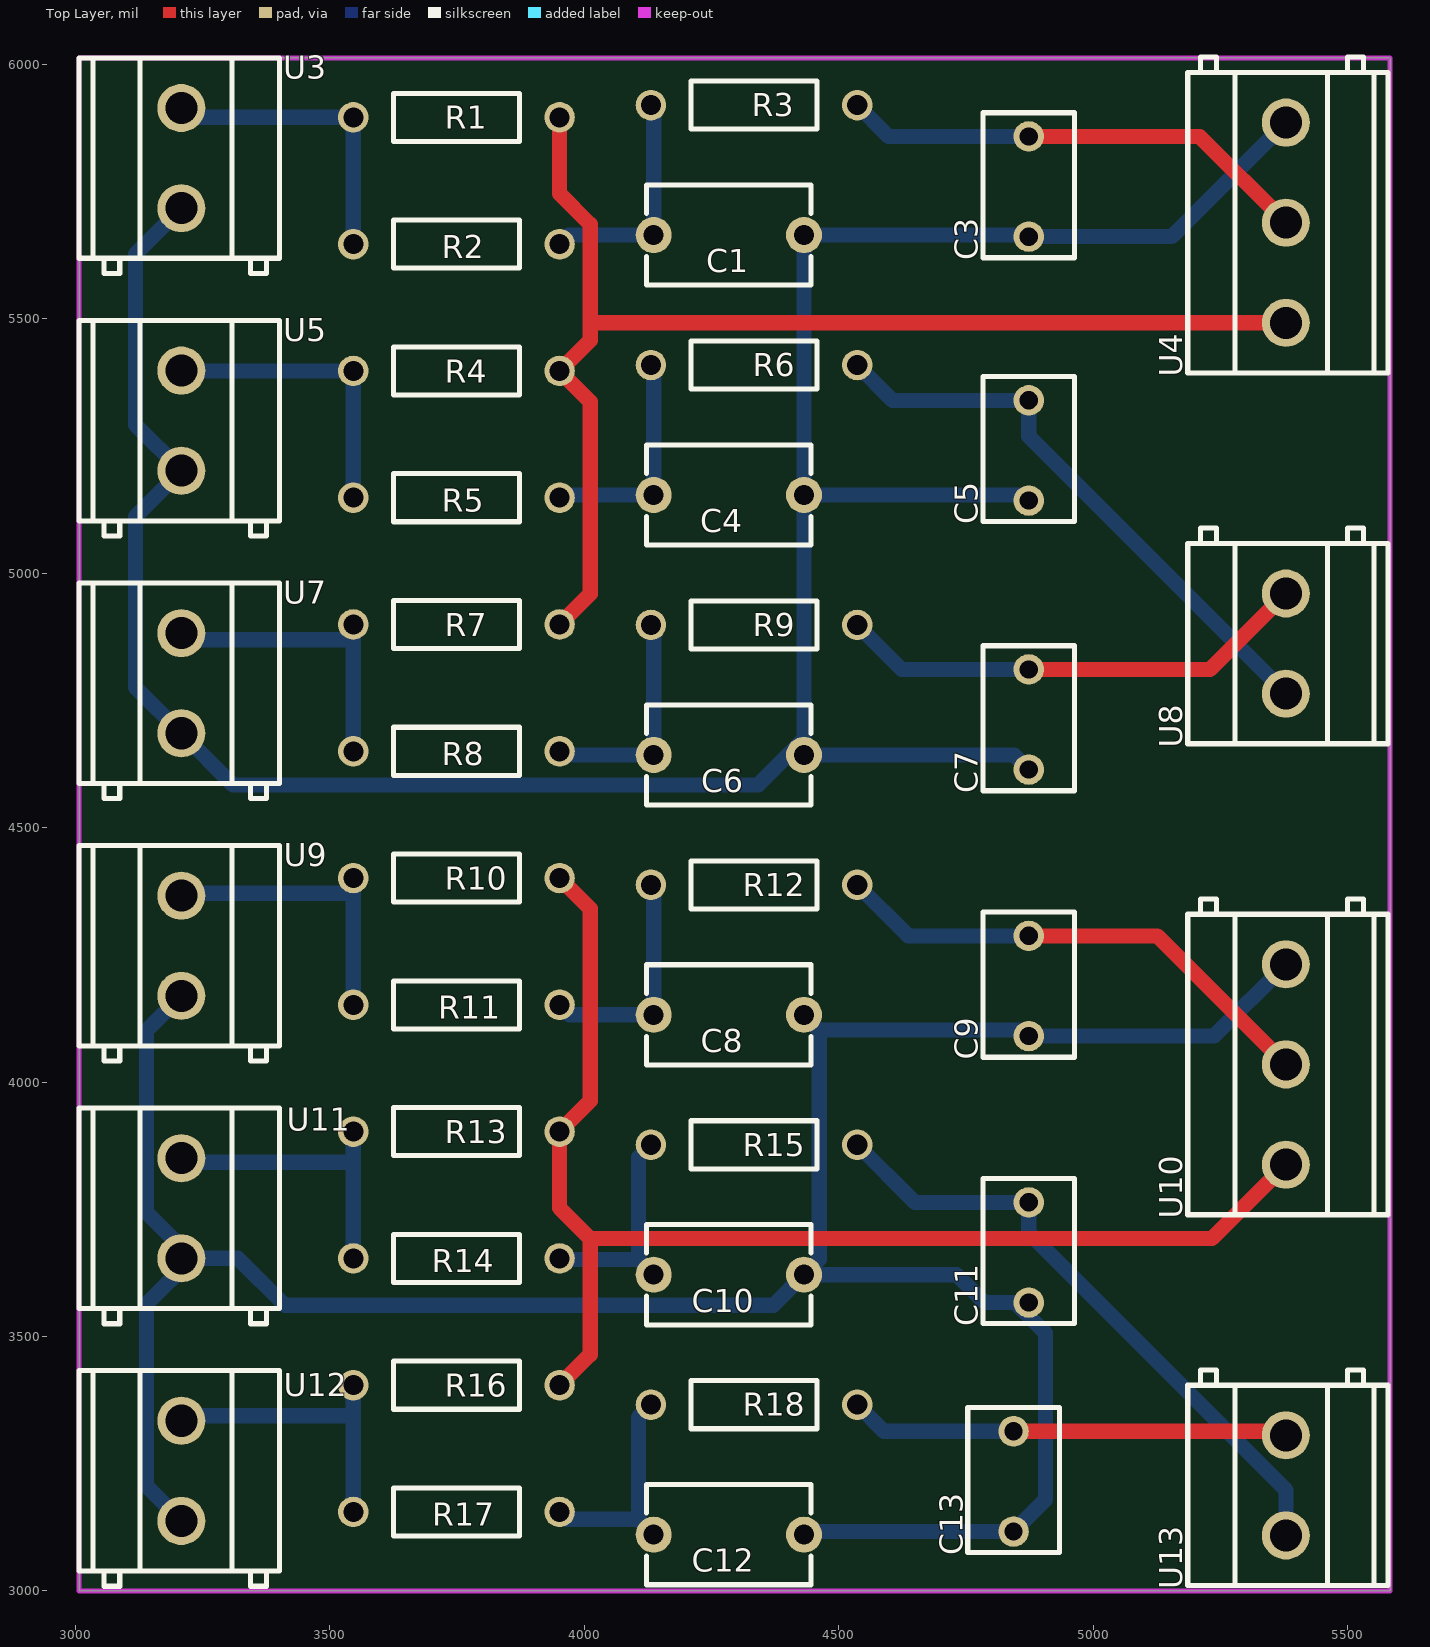
[diagram p0: Top Layer view]
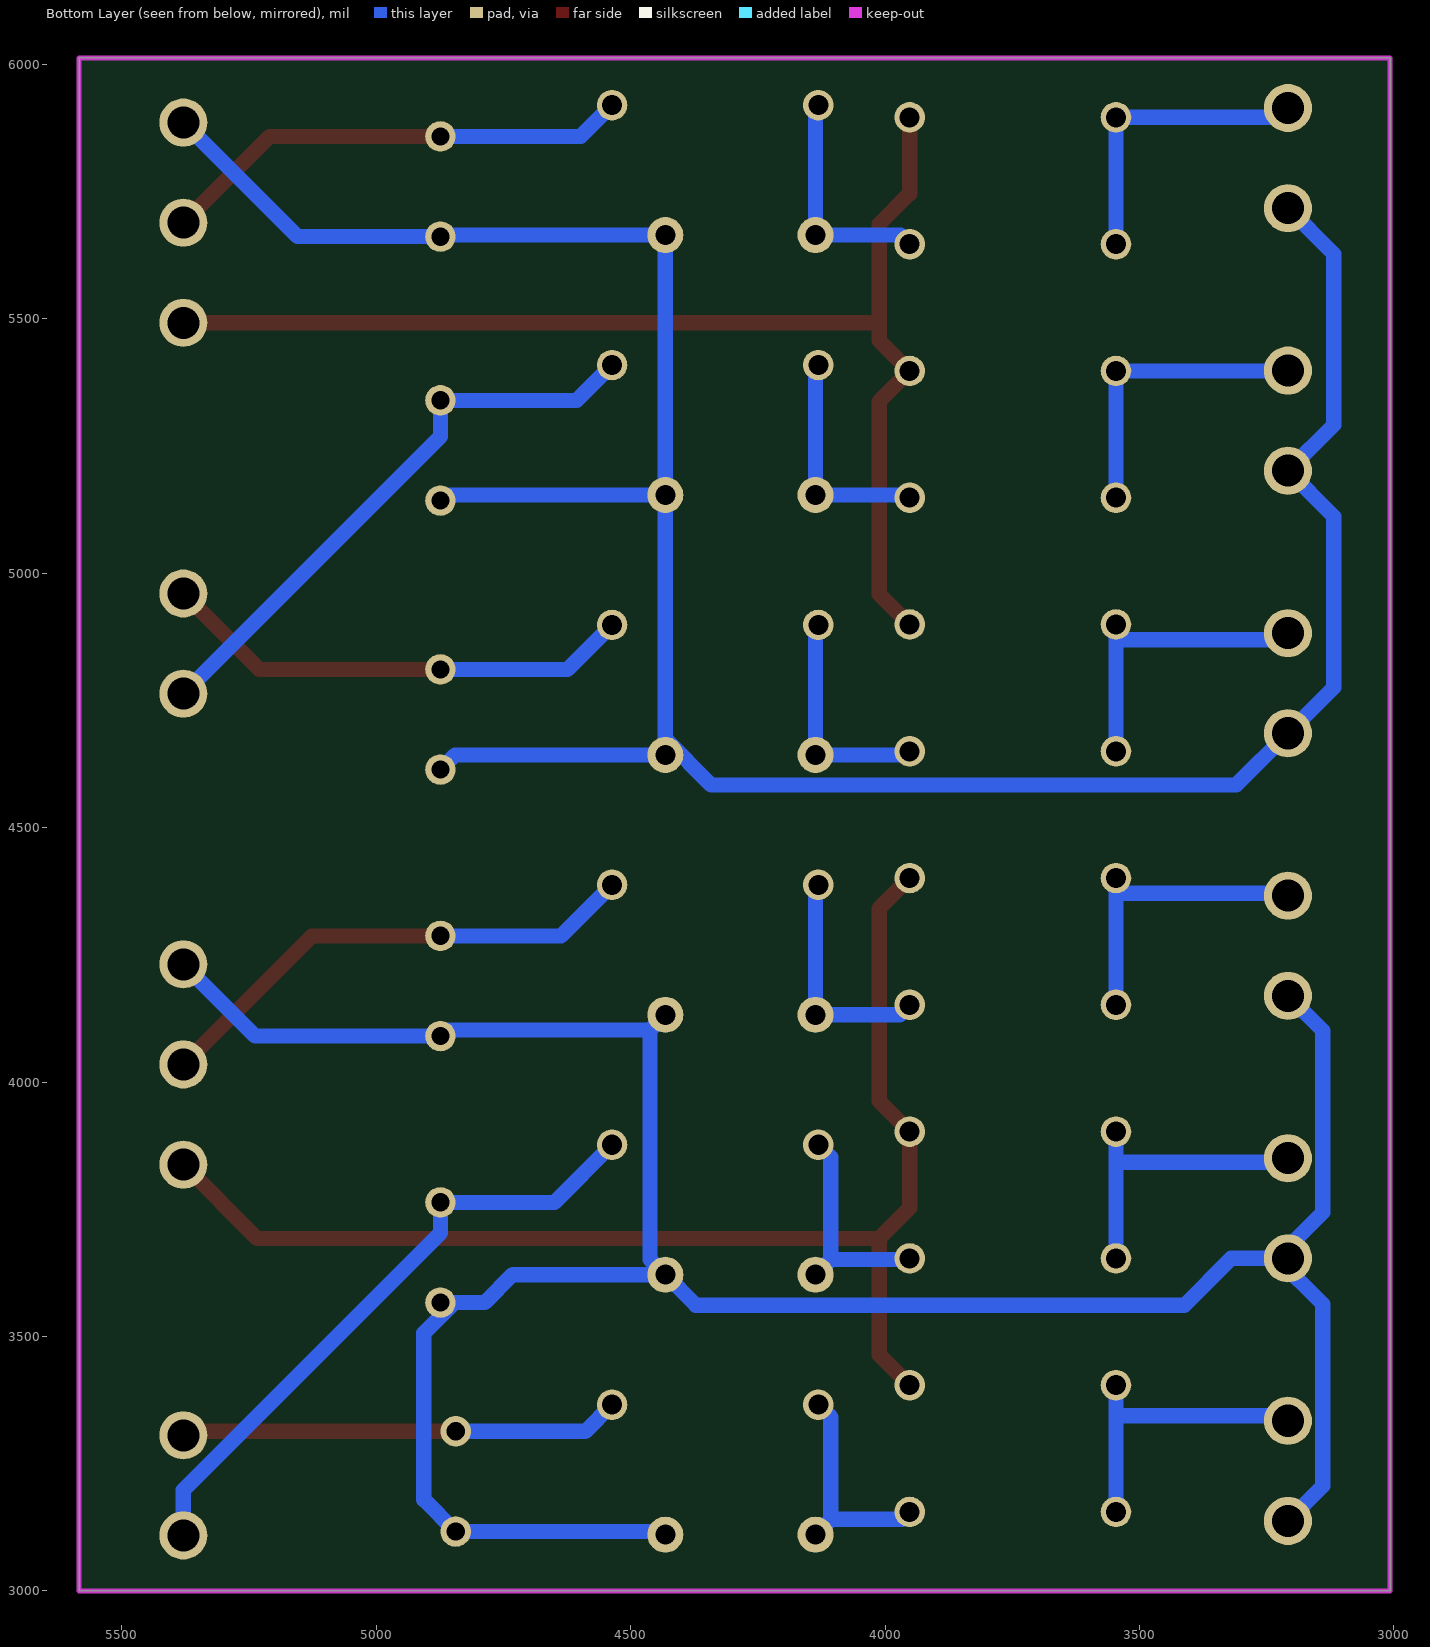
[diagram p1: Bottom Layer view, seen from below]
# Altium PCB MISC52125.pcbdoc
Units mil, origin at the board's own origin, x right, y up, seen from the top; angles counter-clockwise.
Board outline 2576.47 x 3012.76 mil, 2 copper layers (Top Layer, Bottom Layer), stack 62.206 mil thick; 40 components, 22 nets, 82 pads, 0 vias.

## Layer stack, top to bottom
Top Solder Mask Layer: solder mask 0.394, Dk 3.3
Top Layer: signal copper 1.379
Dielectric1: surface 59.449, FR4, Dk 4.5
Bottom Layer: signal copper 1.378
Bottom Solder Mask Layer: solder mask 0.394, Dk 3.3

## Board outline
3007.37,6012.76 3007.37,3000 5583.84,3000 5583.84,6012.76

## Design rules (kind name [scope] priority, off if disabled: settings)
BoardOutlineClearance copperThickness2oz_1 [All] p2 off: genericclearance=7.99 ignorepadtopadclearanceinfootprint=FALSE except(0: Arc-SplitContinuation Track-SplitContinuation SMDPad-SplitContinuation THPad-SplitContinuation Via-SplitContinuation Fill-SplitContinuation Region-SplitContinuation Poly-SplitContinuation Text-SplitContinuation Hole-SplitContinuation; 5.98: Arc-CutoutEdge Track-CutoutEdge SMDPad-CutoutEdge THPad-CutoutEdge Via-CutoutEdge Text-CutoutEdge; 6.89: Hole-OutlineEdge Hole-CutoutEdge; 10: Poly-OutlineEdge Poly-CutoutEdge; 11.81: Arc-OutlineEdge Track-OutlineEdge SMDPad-OutlineEdge THPad-OutlineEdge Via-OutlineEdge Fill-OutlineEdge Region-OutlineEdge Text-OutlineEdge Fill-CutoutEdge Region-CutoutEdge)
BoardOutlineClearance Plane_innerPlane_1 [All] p4 off: genericclearance=4.02 ignorepadtopadclearanceinfootprint=FALSE except(0: Arc-SplitContinuation Track-SplitContinuation SMDPad-SplitContinuation THPad-SplitContinuation Via-SplitContinuation Fill-SplitContinuation Region-SplitContinuation Poly-SplitContinuation Text-SplitContinuation Hole-SplitContinuation; 5.98: Arc-CutoutEdge Track-CutoutEdge SMDPad-CutoutEdge THPad-CutoutEdge Via-CutoutEdge Text-CutoutEdge; 6.89: Hole-OutlineEdge Hole-CutoutEdge; 10: Poly-OutlineEdge Poly-CutoutEdge; 11.81: Arc-OutlineEdge Track-OutlineEdge SMDPad-OutlineEdge THPad-OutlineEdge Via-OutlineEdge Fill-OutlineEdge Region-OutlineEdge Text-OutlineEdge Fill-CutoutEdge Region-CutoutEdge)
BoardOutlineClearance Copper_copperRegion_1 [All] p6 off: genericclearance=4.02 ignorepadtopadclearanceinfootprint=FALSE except(0: Arc-SplitContinuation Track-SplitContinuation SMDPad-SplitContinuation THPad-SplitContinuation Via-SplitContinuation Fill-SplitContinuation Region-SplitContinuation Poly-SplitContinuation Text-SplitContinuation Hole-SplitContinuation; 5.98: Arc-CutoutEdge Track-CutoutEdge SMDPad-CutoutEdge THPad-CutoutEdge Via-CutoutEdge Text-CutoutEdge; 6.89: Hole-OutlineEdge Hole-CutoutEdge; 10: Poly-OutlineEdge Poly-CutoutEdge; 11.81: Arc-OutlineEdge Track-OutlineEdge SMDPad-OutlineEdge THPad-OutlineEdge Via-OutlineEdge Fill-OutlineEdge Region-OutlineEdge Text-OutlineEdge Fill-CutoutEdge Region-CutoutEdge)
BoardOutlineClearance copperThickness1oz_1 [All] p8: genericclearance=4.02 ignorepadtopadclearanceinfootprint=FALSE except(0: Arc-SplitContinuation Track-SplitContinuation SMDPad-SplitContinuation THPad-SplitContinuation Via-SplitContinuation Fill-SplitContinuation Region-SplitContinuation Poly-SplitContinuation Text-SplitContinuation Hole-SplitContinuation; 5.98: Arc-CutoutEdge Track-CutoutEdge SMDPad-CutoutEdge THPad-CutoutEdge Via-CutoutEdge Text-CutoutEdge; 6.89: Hole-OutlineEdge Hole-CutoutEdge; 10: Poly-OutlineEdge Poly-CutoutEdge; 11.81: Arc-OutlineEdge Track-OutlineEdge SMDPad-OutlineEdge THPad-OutlineEdge Via-OutlineEdge Fill-OutlineEdge Region-OutlineEdge Text-OutlineEdge Fill-CutoutEdge Region-CutoutEdge)
Clearance copperThickness2oz [All] p1 off: gap=7.99 ignorepadtopadclearanceinfootprint=FALSE except(5.98: SMDPad-Track SMDPad-SMDPad THPad-Track SMDPad-THPad THPad-THPad Track-Via SMDPad-Via THPad-Via Via-Via Fill-SMDPad Region-SMDPad Fill-THPad Region-THPad Fill-Via Region-Via Fill-Fill Fill-Region Region-Region Arc-Track Arc-SMDPad Arc-THPad Arc-Via Fill-Arc Region-Arc Arc-Arc Text-Track SMDPad-Text Text-THPad Text-Via Fill-Text Region-Text Arc-Text Text-Text; 6.89: Hole-Track Hole-SMDPad Hole-THPad Hole-Via Fill-Hole Region-Hole Hole-Arc Hole-Text; 10: Poly-Track Poly-SMDPad Poly-THPad Poly-Via Poly-Fill Poly-Region Poly-Poly Poly-Arc Poly-Text Poly-Hole; 11.81: Fill-Track Region-Track)
Clearance Plane_innerPlane [All] p3 off: gap=4.02 ignorepadtopadclearanceinfootprint=FALSE except(5.98: SMDPad-Track SMDPad-SMDPad THPad-Track SMDPad-THPad THPad-THPad Track-Via SMDPad-Via THPad-Via Via-Via Fill-SMDPad Region-SMDPad Fill-THPad Region-THPad Fill-Via Region-Via Fill-Fill Fill-Region Region-Region Arc-Track Arc-SMDPad Arc-THPad Arc-Via Fill-Arc Region-Arc Arc-Arc Text-Track SMDPad-Text Text-THPad Text-Via Fill-Text Region-Text Arc-Text Text-Text; 6.89: Hole-Track Hole-SMDPad Hole-THPad Hole-Via Fill-Hole Region-Hole Hole-Arc Hole-Text; 10: Poly-Track Poly-SMDPad Poly-THPad Poly-Via Poly-Fill Poly-Region Poly-Poly Poly-Arc Poly-Text Poly-Hole; 11.81: Fill-Track Region-Track)
Clearance Copper_copperRegion [All] p5 off: gap=4.02 ignorepadtopadclearanceinfootprint=FALSE except(5.98: SMDPad-Track SMDPad-SMDPad THPad-Track SMDPad-THPad THPad-THPad Track-Via SMDPad-Via THPad-Via Via-Via Fill-SMDPad Region-SMDPad Fill-THPad Region-THPad Fill-Via Region-Via Fill-Fill Fill-Region Region-Region Arc-Track Arc-SMDPad Arc-THPad Arc-Via Fill-Arc Region-Arc Arc-Arc Text-Track SMDPad-Text Text-THPad Text-Via Fill-Text Region-Text Arc-Text Text-Text; 6.89: Hole-Track Hole-SMDPad Hole-THPad Hole-Via Fill-Hole Region-Hole Hole-Arc Hole-Text; 10: Poly-Track Poly-SMDPad Poly-THPad Poly-Via Poly-Fill Poly-Region Poly-Poly Poly-Arc Poly-Text Poly-Hole; 11.81: Fill-Track Region-Track)
Clearance copperThickness1oz [All] p7: gap=4.02 ignorepadtopadclearanceinfootprint=FALSE except(5.98: SMDPad-Track SMDPad-SMDPad THPad-Track SMDPad-THPad THPad-THPad Track-Via SMDPad-Via THPad-Via Via-Via Fill-SMDPad Region-SMDPad Fill-THPad Region-THPad Fill-Via Region-Via Fill-Fill Fill-Region Region-Region Arc-Track Arc-SMDPad Arc-THPad Arc-Via Fill-Arc Region-Arc Arc-Arc Text-Track SMDPad-Text Text-THPad Text-Via Fill-Text Region-Text Arc-Text Text-Text; 6.89: Hole-Track Hole-SMDPad Hole-THPad Hole-Via Fill-Hole Region-Hole Hole-Arc Hole-Text; 10: Poly-Track Poly-SMDPad Poly-THPad Poly-Via Poly-Fill Poly-Region Poly-Poly Poly-Arc Poly-Text Poly-Hole; 11.81: Fill-Track Region-Track)
DiffPairsRouting differentialPair [All] p1: maxlimit=6 minlimit=6 mostfreqgap=6 toplayer_minwidth=5 toplayer_prefwidth=10 toplayer_maxwidth=100 toplayer_mingap=6 toplayer_prefgap=6 toplayer_maxgap=6 bottomlayer_minwidth=5 bottomlayer_prefwidth=10 bottomlayer_maxwidth=100 bottomlayer_mingap=6 bottomlayer_prefgap=6 bottomlayer_maxgap=6 maxuncoupledlength=10
HoleToHoleClearance otherClearance [All] p1: gap=11.81 allowstackedmicrovias=TRUE
Length netLength [All] p1: minlimit=0 maxlimit=0
PasteMaskExpansion pasteMaskExpansion [All] p1: expansion=0
PlaneConnect innerPlane [All] p1: planeconnectstyle=Relief reliefexpansion=20 reliefentries=4 reliefconductorwidth=10 reliefairgap=10
PolygonConnect copperRegion [All] p1: connectstyle=Relief reliefconductorwidth=10 reliefentries=4 polygonreliefangle="90 Angle" airgapwidth=10 via.connectstyle=Relief via.reliefconductorwidth=10 via.reliefentries=4 via.polygonreliefangle="90 Angle" via.airgapwidth=10
RoutingVias viaSize [All] p1: holewidth=12.01 width=24.02 viastyle="Through Hole" minholewidth=11.81 minwidth=19.68 maxholewidth=248.03 maxwidth=393.7
SolderMaskExpansion solderMaskExpansion [IsVia] p1: expansion=-1000 istentingtop=TRUE
SolderMaskExpansion solderMaskExpansion [All] p2: expansion=2.01 istentingtop=FALSE
Width copperThickness2oz_2 [All] p1 off: maxlimit=100 minlimit=8 preferedwidth=10
Width copperThickness1oz_2 [All] p2: maxlimit=100 minlimit=5 preferedwidth=30

## Components (designator, comment, footprint, x,y, rotation, side; value= is the part's Value field where it differs from the comment)
C1 "2.2nF" CAP-TH_L8.0-W5.0-P7.50-D1.0 4284.15,5664.58 r180 top
C3 "220pF" CAP-TH_L7.2-W4.5-P5.00-D0.5 4873.84,5760 r90 top
C4 "2.2nF" CAP-TH_L8.0-W5.0-P7.50-D1.0 4284.15,5153.75 r180 top
C5 "220pF" CAP-TH_L7.2-W4.5-P5.00-D0.5 4873.84,5241.26 r90 top
C6 "2.2nF" CAP-TH_L8.0-W5.0-P7.50-D1.0 4284.15,4642.92 r180 top
C7 "220pF" CAP-TH_L7.2-W4.5-P5.00-D0.5 4873.84,4712.5 r90 top
C8 "2.2nF" CAP-TH_L8.0-W5.0-P7.50-D1.0 4284.15,4132.09 r180 top
C9 "220pF" CAP-TH_L7.2-W4.5-P5.00-D0.5 4873.84,4188.75 r90 top
C10 "2.2nF" CAP-TH_L8.0-W5.0-P7.50-D1.0 4284.15,3621.26 r180 top
C11 "220pF" CAP-TH_L7.2-W4.5-P5.00-D0.5 4873.84,3665 r90 top
C12 "2.2nF" CAP-TH_L8.0-W5.0-P7.50-D1.0 4284.15,3110.43 r180 top
C13 "220pF" CAP-TH_L7.2-W4.5-P5.00-D0.5 4843.84,3215 r90 top
R1 "51kΩ" Res_1/4W 3748.84,5895.91 r0 top
R2 "390Ω" Res_1/4W 3748.84,5646.73 r180 top
R3 "3.6kΩ" Res_1/4W 4333.84,5920 r180 top
R4 "51kΩ" Res_1/4W 3748.84,5397.56 r0 top
R5 "390Ω" Res_1/4W 3748.84,5148.39 r180 top
R6 "3.6kΩ" Res_1/4W 4333.84,5409.17 r180 top
R7 "51kΩ" Res_1/4W 3748.84,4899.21 r0 top
R8 "390Ω" Res_1/4W 3748.84,4650.04 r180 top
R9 "3.6kΩ" Res_1/4W 4333.84,4898.34 r180 top
R10 "51kΩ" Res_1/4W 3748.84,4400.87 r0 top
R11 "390Ω" Res_1/4W 3748.84,4151.69 r180 top
R12 "3.6kΩ" Res_1/4W 4333.84,4387.51 r180 top
R13 "51kΩ" Res_1/4W 3748.84,3902.52 r0 top
R14 "390Ω" Res_1/4W 3748.84,3653.35 r180 top
R15 "3.6kΩ" Res_1/4W 4333.84,3876.68 r180 top
R16 "51kΩ" Res_1/4W 3748.84,3404.17 r0 top
R17 "390Ω" Res_1/4W 3748.84,3155 r180 top
R18 "3.6kΩ" Res_1/4W 4333.84,3365.85 r180 top
U3 "KF128L-5.0-2P" CONN-TH_P5.00_KF128L-5.0-2P 3208.15,5815.91 r270 top
U4 "KF128L-5.0-3P" CONN-TH_3P-P5.00_KF128L-5.0-3P 5379.05,5688.94 r90 top
U5 "KF128L-5.0-2P" CONN-TH_P5.00_KF128L-5.0-2P 3208.15,5299.88 r270 top
U7 "KF128L-5.0-2P" CONN-TH_P5.00_KF128L-5.0-2P 3208.15,4783.86 r270 top
U8 "KF128L-5.0-2P" CONN-TH_P5.00_KF128L-5.0-2P 5379.05,4861.71 r90 top
U9 "KF128L-5.0-2P" CONN-TH_P5.00_KF128L-5.0-2P 3208.15,4267.83 r270 top
U10 "KF128L-5.0-3P" CONN-TH_3P-P5.00_KF128L-5.0-3P 5379.05,4034.48 r90 top
U11 "KF128L-5.0-2P" CONN-TH_P5.00_KF128L-5.0-2P 3208.15,3751.81 r270 top
U12 "KF128L-5.0-2P" CONN-TH_P5.00_KF128L-5.0-2P 3208.15,3235.79 r270 top
U13 "KF128L-5.0-2P" CONN-TH_P5.00_KF128L-5.0-2P 5379.05,3207.24 r90 top

## Footprints (in the part's own frame and the unit in brackets; to place one, negate y for a bottom-side part, rotate by r counter-clockwise, add the part's x,y. Pads: shape width x height; smd on the part's side, far side on the other; paste and mask are expansions set on the pad)
CAP-TH_L7.2-W4.5-P5.00-D0.5 [mil]
  round 60 hole 36 paste+0 mask+1.97: 1(-98.43,0) 2(98.43,0)
  silkscreen extent -140,-90 145,90
CAP-TH_L8.0-W5.0-P7.50-D1.0 [mm]
  round 1.8 hole 1: 1(-3.75,0) 2(3.75,0)
  silkscreen extent -4.1,-2.5 4.1,2.5
CONN-TH_3P-P5.00_KF128L-5.0-3P [mm]
  round 2.4 hole 1.6: 1(-5,0) 2(0,0) 3(5,0)
  silkscreen extent -7.5,-5.1 8.26,4.9
CONN-TH_P5.00_KF128L-5.0-2P [mm]
  round 2.4 hole 1.6: 1(-2.5,0) 2(2.5,0)
  silkscreen extent -5,-5.1 5.76,4.9
Res_1/4W [mil]
  round 60 hole 39.37 paste+0 mask+2: 1(-202.76,0) 2(202.76,0)
  silkscreen extent -124,-47 124,47

## Nets (pads, with @x,y where several pads share a name; then routed paths per layer and width w, separated by ;. In a path a pad name is that pad's centre, name@x,y a point inside that pad or via, vN(x,y) a via of type N, cw(c..) or ccw(c..) an arc to the next point about the centre after c; other vN are vias at no path point)
$1N473: R1.1 R2.2 U3.1 | length 594.7
  Bottom Layer w30: U3.1 3226.58,5895.91 R1.1 R2.2
$1N545: C1.2 R2.1 R3.2 | length 450
  Bottom Layer w30: R2.1 3969.45,5664.58 C1.2 4136.51,5914.57 R3.2
$1N788: C3.2 R3.1 U4.2 | length 938.2
  Top Layer w30: C3.2 5209.57,5858.43 U4.2
  Bottom Layer w30: R3.1 4598.18,5858.43 C3.2
$1N825: R1.2 R4.2 R7.2 U4.1 | length 2463.6
  Top Layer w30: R7.2 4011.6,4959.21 4011.6,5337.56 R4.2 4011.6,5457.56 4011.6,5492.09 ; R1.2 3951.6,5745.91 4011.6,5685.91 4011.6,5492.09 ; U4.1 4011.6,5492.09
$1N1139: R4.1 R5.2 U5.1 | length 587.4
  Bottom Layer w30: U5.1 3208.9,5397.56 R4.1 R5.2
$1N1142: C4.2 R5.1 R6.2 | length 444.8
  Bottom Layer w30: R5.1 3956.97,5153.75 C4.2 4136.51,5403.74 R6.2
$1N1144: C5.2 R6.1 U8.1 | length 1151.7
  Bottom Layer w30: R6.1 4606.09,5339.69 C5.2 4873.84,5268.49 U8.1
$1N1393: R7.1 R8.2 U7.1 | length 592.5
  Bottom Layer w30: U7.1 3221.22,4869.21 3546.08,4869.21 ; R8.2 3546.08,4869.21 ; R7.1 3546.08,4869.21
$1N1396: C6.2 R8.1 R9.2 | length 445.5
  Bottom Layer w30: R8.1 3958.72,4642.92 C6.2 4136.51,4892.91 R9.2
$1N1398: C7.2 R9.1 U8.2 | length 940.5
  Top Layer w30: C7.2 5229.84,4810.93 U8.2
  Bottom Layer w30: R9.1 4624.02,4810.93 C7.2
$1N2154: R10.1 R11.2 U9.1 | length 589
  Bottom Layer w30: U9.1 3212.76,4370.87 3546.08,4370.87 ; R11.2 3546.08,4370.87 ; R10.1 3546.08,4370.87
$1N2157: C8.2 R11.1 R12.2 | length 450.7
  Bottom Layer w30: R11.1 3971.2,4132.09 C8.2 4136.51,4382.08 R12.2
$1N2159: C9.2 R12.1 U10.2 | length 988.7
  Top Layer w30: C9.2 5126.35,4287.18 U10.2
  Bottom Layer w30: R12.1 4636.93,4287.18 C9.2
$1N2166: R10.2 R13.2 R16.2 U10.1 | length 2523.7
  Top Layer w30: R16.2 4011.6,3464.17 4011.6,3692.52 ; R10.2 4011.6,4340.87 4011.6,3962.52 R13.2 3951.6,3752.52 4011.6,3692.52 ; U10.1 5233.94,3692.52 4011.6,3692.52
$1N2177: R13.1 R14.2 U11.1 | length 590.3
  Bottom Layer w30: U11.1 3215.87,3842.52 3546.08,3842.52 ; R14.2 3546.08,3842.52 ; R13.1 3546.08,3842.52
$1N2180: C10.2 R14.1 R15.2 | length 433.8
  Bottom Layer w30: R14.1 3953.68,3651.26 4106.51,3651.26 ; R15.2 4106.51,3852.11 4106.51,3651.26 ; C10.2 4106.51,3651.26
$1N2182: C11.2 R15.1 U13.1 | length 1248
  Bottom Layer w30: R15.1 4649.85,3763.43 C11.2 4873.84,3703.43 5379.05,3198.22 U13.1
$1N2191: R16.1 R17.2 U12.1 | length 591.2
  Bottom Layer w30: U12.1 3218.12,3344.17 3546.08,3344.17 ; R17.2 3546.08,3344.17 ; R16.1 3546.08,3344.17
$1N2194: C12.2 R17.1 R18.2 | length 439
  Bottom Layer w30: R17.1 3966.17,3140.43 4106.51,3140.43 ; R18.2 4106.51,3341.28 4106.51,3140.43 ; C12.2 4106.51,3140.43
$1N2196: C13.2 R18.1 U13.2 | length 867.4
  Top Layer w30: C13.2 5371.29,3313.43 U13.2
  Bottom Layer w30: R18.1 4589.02,3313.43 C13.2
AGND: C8.1 C9.1 C10.1 C11.1 C12.1 C13.1 U9.2 U10.3 U11.2 U12.2 | length 5346.3
  Bottom Layer w30: U12.2 3139.67,3205.84 3139.67,3563.39 U11.2@3229.67,3653.39 ; U11.2 U11.2@3229.67,3653.39 ; U9.2 3139.67,4100.93 3139.67,3743.39 U11.2@3229.67,3653.39 ; C12.1 4437.94,3116.57 C13.1 4906.48,3179.22 4906.48,3506.57 C11.1@4846.48,3566.57 ; C8.1 4461.79,4102.09 ; C11.1 C11.1@4846.48,3566.57 ; U10.3 5238.04,4090.32 C9.1 4862.07,4102.09 4461.79,4102.09 ; U11.2@3229.67,3653.39 3319.67,3653.39 3411.79,3561.26 4371.79,3561.26 C10.1 ; C10.1 4461.79,3651.26 4461.79,4102.09 ; C10.1 4731.79,3621.26 4786.48,3566.57 C11.1@4846.48,3566.57
GND: C1.1 C3.1 C4.1 C5.1 C6.1 C7.1 U3.2 U4.3 U5.2 U7.2 | length 5447.8
  Bottom Layer w30: U3.2 3118.15,5627.48 3118.15,5291.46 U5.2 3118.15,5111.46 3118.15,4775.43 U7.2 3309.83,4583.75 4341.79,4583.75 C6.1@4431.79,4673.75 ; C7.1 4844.99,4642.92 C6.1 C6.1@4431.79,4673.75 ; C5.1 4862.92,5153.75 C4.1 ; U4.3 5154.83,5661.57 C3.1 4870.83,5664.58 C1.1 C4.1 ; C6.1@4431.79,4673.75 C4.1

## Keep-outs
Board Outline Layer:
  the board outline again, w10